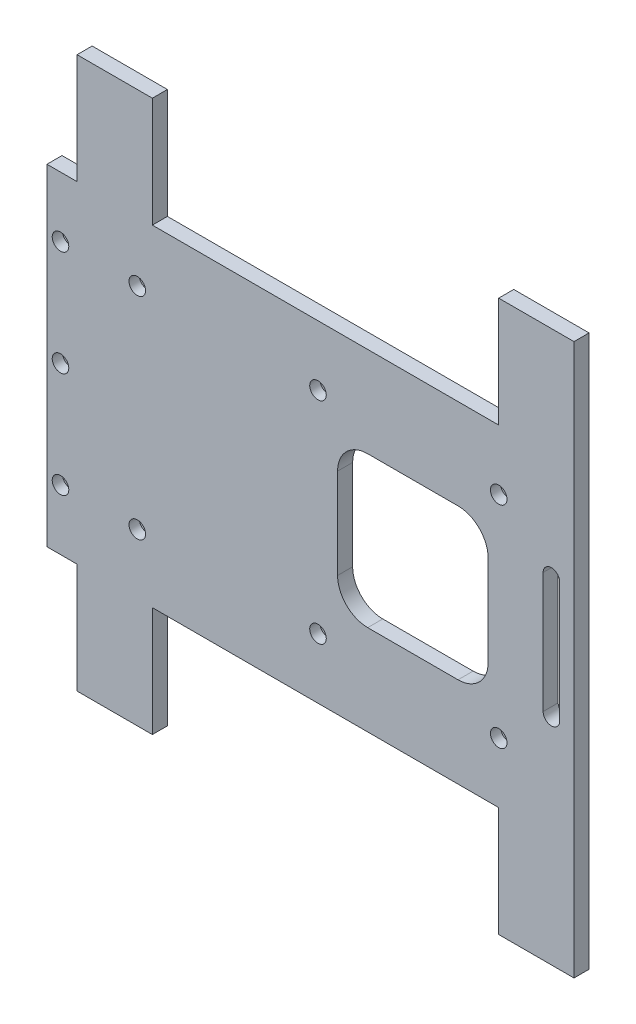
from build123d import *

# Parameters (mm, degrees)
SKETCH_1_W                = 350
SKETCH_1_H                = 220
EXTRUDE_1_DEPTH           = 5
CUT_EXTRUDE_1_DEPTH       = 207.942020866
CUT_EXTRUDE_2_DEPTH       = 207.942020866
HOLE_WIZARD_1_D           = 6.6
HOLE_WIZARD_1_DEPTH       = 15
HOLE_WIZARD_1_CBORE_D     = 11
HOLE_WIZARD_1_CBORE_DEPTH = 6.8
HOLE_WIZARD_1_TIP         = 1.982840043
SKETCH_8_W                = 50
SKETCH_8_H                = 73
EXTRUDE_2_DEPTH           = 10
PATTERN_LINEAR_1_COUNT    = 2
PATTERN_LINEAR_1_PITCH    = 280


with BuildPart() as part:
    # 草图1 → 凸台-拉伸1 (new, symmetric)
    with BuildSketch(Plane.XY):
        Rectangle(SKETCH_1_W, SKETCH_1_H)
    extrude(amount=EXTRUDE_1_DEPTH, both=True)

    # 草图2 → 切除-拉伸1 (cut, through all)
    with BuildSketch(Plane.XY.offset(5)):
        with BuildLine():
            Line((-208, 40), (-208, -40))
            ThreePointArc((-208, -40), (-213.5, -45.5), (-219, -40))
            Line((-219, -40), (-219, 40))
            ThreePointArc((-219, 40), (-213.5, 45.5), (-208, 40))
        make_face()
        with BuildLine():
            Line((165.5, 40), (165.5, -40))
            ThreePointArc((165.5, -40), (160, -45.5), (154.5, -40))
            Line((154.5, -40), (154.5, 40))
            ThreePointArc((154.5, 40), (160, 45.5), (165.5, 40))
        make_face()
    extrude(amount=-CUT_EXTRUDE_1_DEPTH, mode=Mode.SUBTRACT)

    # 草图6 → 切除-拉伸2 (cut, through all)
    with BuildSketch(Plane.XY.offset(5)):
        with BuildLine():
            Line((98, -50), (38, -50))
            ThreePointArc((38, -50), (23.857864376, -44.142135624), (18, -30))
            Line((18, -30), (18, 30))
            ThreePointArc((18, 30), (23.857864376, 44.142135624), (38, 50))
            Line((38, 50), (98, 50))
            ThreePointArc((98, 50), (112.142135624, 44.142135624), (118, 30))
            Line((118, 30), (118, -30))
            ThreePointArc((118, -30), (112.142135624, -44.142135624), (98, -50))
        make_face()
    extrude(amount=-CUT_EXTRUDE_2_DEPTH, mode=Mode.SUBTRACT)

    # 打孔尺寸(%根据)内六角圆柱头螺钉的类型1
    with Locations(Plane(origin=(-115, 70, 5), x_dir=(1, 0, 0), z_dir=(0, 0, 1))):
        with Locations((0, 0), (0, -140), (-51, 0), (-51, -140), (-51, -70), (120, 0), (240, 0), (240, -140), (120, -140)):
            CounterBoreHole(HOLE_WIZARD_1_D / 2, HOLE_WIZARD_1_CBORE_D / 2, HOLE_WIZARD_1_CBORE_DEPTH, depth=HOLE_WIZARD_1_DEPTH)
            with Locations((0, 0, -(HOLE_WIZARD_1_DEPTH + HOLE_WIZARD_1_TIP / 2))):  # 118° drill point
                Cone(0, HOLE_WIZARD_1_D / 2, HOLE_WIZARD_1_TIP, mode=Mode.SUBTRACT)

    # 草图8 → 凸台-拉伸2 (add)
    with BuildSketch(Plane(origin=(0, 0, -5), x_dir=(-1, 0, 0), z_dir=(0, 0, -1))):
        with Locations((-150, 146.5)):
            Rectangle(SKETCH_8_W, SKETCH_8_H)
        with Locations((-150, -146.5)):
            Rectangle(SKETCH_8_W, SKETCH_8_H)
    extrude_2 = extrude(amount=-EXTRUDE_2_DEPTH)

    # 阵列(线性)1: 凸台-拉伸2 ×2
    with Locations(*[(-i * PATTERN_LINEAR_1_PITCH, 0, 0) for i in range(1, PATTERN_LINEAR_1_COUNT)]):
        add(extrude_2)


solid = part.part
